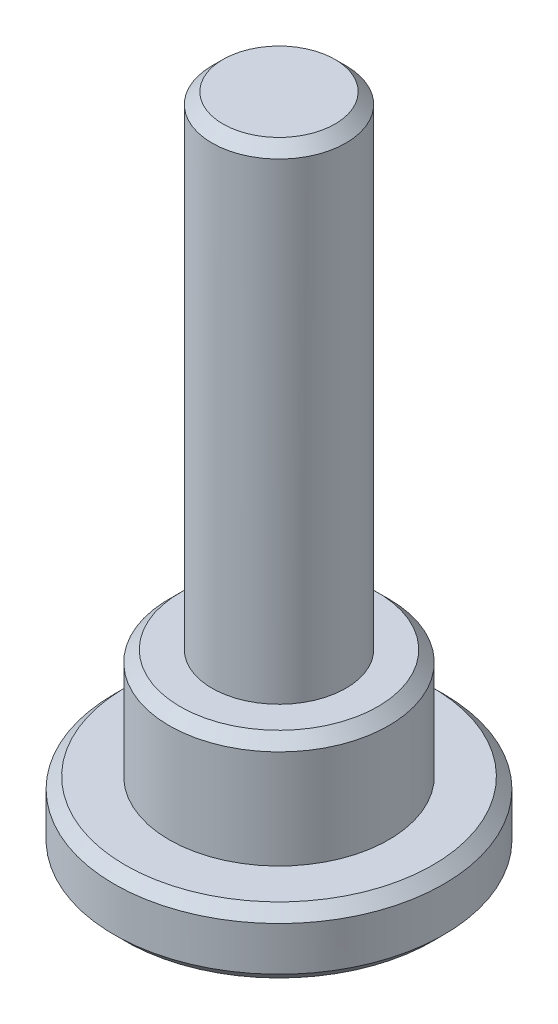
SolidWorks part; units mm, degrees
material "20#"
ref_plane "Front Plane" through (0, 0, 0) normal (0, 0, 1) x (1, 0, 0)
ref_plane "Top Plane" through (0, 0, 0) normal (0, 1, 0) x (1, 0, 0)
ref_plane "Right Plane" through (0, 0, 0) normal (1, 0, 0) x (0, 0, -1)
sketch "Sketch1" plane through (0, 0, 0) normal (1, 0, 0) x (0, 0, -1)
  line L0 (0, 0) -> (0, 30) construction
  line L1 (0, 30) -> (3.05, 30)
  line L2 (3.05, 30) -> (3.05, 8)
  line L3 (3.05, 8) -> (5, 8)
  line L4 (5, 8) -> (5, 3)
  line L5 (5, 3) -> (7.5, 3)
  line L6 (7.5, 3) -> (7.5, 0)
  line L7 (7.5, 0) -> (0, 0)
  line L8 (0, 0) -> (0, 30)
  dimension "D1" = 6.1
  dimension "D2" = 10
  dimension "D3" = 15
  dimension "D4" = 3
  dimension "D5" = 5
  dimension "D6" = 22
revolve "Revolve1" add sketch "Sketch1" angle 360 about L0
chamfer "Chamfer1" distance 0.5 angle 45 4 edges at (0, 0, -7.5) (0, 3, -7.5) (0, 8, -5) (0, 30, -3.05)
